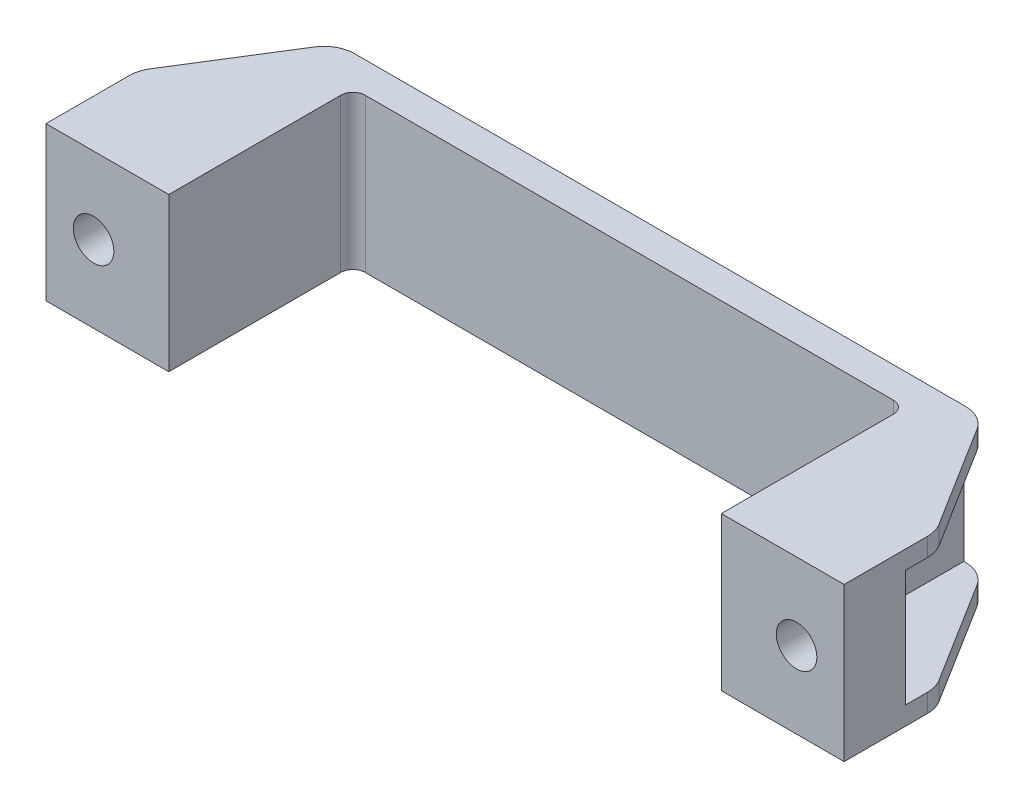
SolidWorks part; units mm, degrees
ref_plane "Frontal" through (0, 0, 0) normal (0, 0, 1) x (1, 0, 0)
ref_plane "Superior" through (0, 0, 0) normal (0, 1, 0) x (1, 0, 0)
ref_plane "Direito" through (0, 0, 0) normal (1, 0, 0) x (0, 0, -1)
sketch "Sketch1" plane through (0, 0, 0) normal (0, 1, 0) x (1, 0, 0)
  line L0 (-52.5, 0) -> (52.5, 0)
  line L1 (52.5, 0) -> (65, -20)
  line L2 (65, -20) -> (65, -35)
  line L3 (65, -35) -> (45, -35)
  line L4 (-65, -35) -> (-65, -20)
  line L5 (-65, -20) -> (-52.5, 0)
  line L6 (-45, -35) -> (-45, -5)
  line L7 (45, -5) -> (45, -35)
  line L8 (-45, -5) -> (45, -5)
  line L9 (-45, -35) -> (-65, -35)
  dimension "D1" = 130
  dimension "D2" = 35
  dimension "D3" = 5
  dimension "D4" = 20
  dimension "D5" = 20
  dimension "D6" = 65
  dimension "D7" = 105
  dimension "D8" = 15
  dimension "D9" = 15
extrude "Boss-Extrude1" add sketch "Sketch1" along normal blind 25
sketch "Sketch2" plane through (0, 0, 0) normal (0, 0, -1) x (-1, 0, 0)
  line L0 (-65, 25) -> (-52.5, 25) construction
  line L1 (-68, 22) -> (-49.5, 22)
  line L2 (-68, 22) -> (-68, 3)
  line L3 (-68, 3) -> (-49.5, 3)
  line L4 (-49.5, 22) -> (-49.5, 3)
  line L5 (68, 22) -> (49.5, 22)
  line L6 (68, 22) -> (68, 3)
  line L7 (68, 3) -> (49.5, 3)
  line L8 (49.5, 22) -> (49.5, 3)
  line L9 (-65, 0) -> (-52.5, 0) construction
  line L10 (-52.5, 25) -> (-52.5, 0) construction
  line L11 (-65, 25) -> (-65, 0) construction
  line L12 (52.5, 25) -> (52.5, 0) construction
  line L13 (65, 25) -> (65, 0) construction
  line L14 (52.5, 25) -> (65, 25) construction
  line L15 (52.5, 0) -> (65, 0) construction
  dimension "D1" = 3
  dimension "D2" = 3
  dimension "D3" = 3
  dimension "D4" = 3
  dimension "D5" = 3
  dimension "D6" = 3
  dimension "D7" = 3
  dimension "D8" = 3
extrude "Cut-Extrude1" cut sketch "Sketch2" against normal blind 25
hole_wizard "Counterbore for pan head screw of M61" positions "Sketch4" profile "Sketch3" counterbore size "M6" standard "ISO" end condition through all
sketch "Sketch4" plane through (0, 0, 25) normal (0, 0, -1) x (-1, 0, 0)
  line L0 (-65, 22) -> (-65, 3) construction
  line L2 (-65, 25) -> (-52.5, 25) construction
  line L3 (52.5, 25) -> (65, 25) construction
  line L4 (65, 22) -> (65, 3) construction
  point P0 (-57.25, 12.5)
  point P2 (57.25, 12.5)
  dimension "D1" = 7.75
  dimension "D2" = 12.5
  dimension "D3" = 12.5
  dimension "D4" = 7.75
sketch "Sketch3" plane through (57.25, 12.5, 25) normal (1, 0, 0) x (0, 1, 0)
  line L0 (0, 0) -> (0, 10)
  line L1 (0, 10) -> (3.3, 10)
  line L3 (3.3, 10) -> (3.3, 4.6)
  line L4 (3.3, 4.6) -> (6.5, 4.6)
  line L5 (6.5, 4.6) -> (6.5, 0)
  line L7 (6.5, 0) -> (0, 0)
  line L11 (0, -6.35) -> (0, 107.95) construction
  dimension "Thru Hole Dia." = 6.6
  dimension "Thru Hole Depth" = 10
  dimension "C'Bore Dia." = 13
  dimension "C'Bore Depth" = 4.6
fillet "Filete1" radius 5 8 edges at (52.5, 1.5, 0) (-52.5, 23.5, 0) (-52.5, 1.5, 0) (-65, 1.5, 20) (-65, 23.5, 20) (65, 1.5, 20) (65, 23.5, 20) (52.5, 23.5, 0)
fillet "Filete2" radius 2 2 edges at (45, 12.5, 5) (-45, 12.5, 5)
